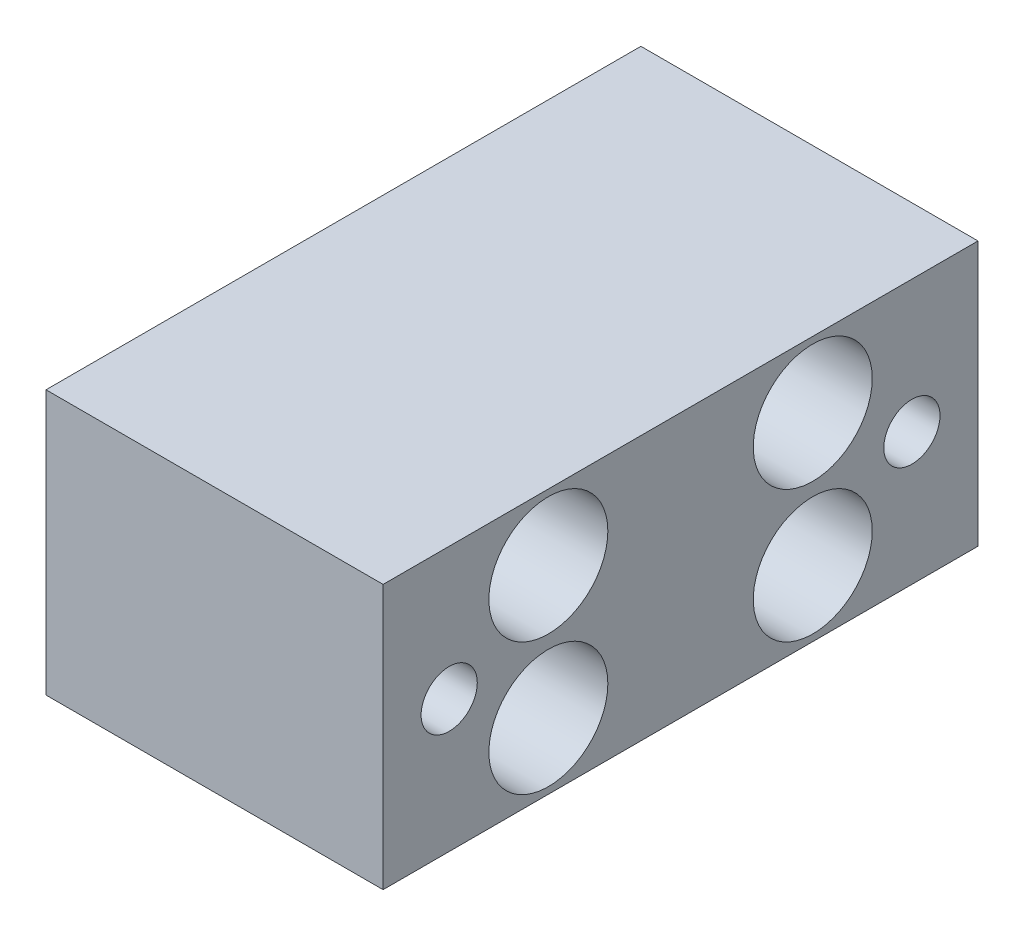
SolidWorks part; units mm, degrees
ref_plane "前视基准面" through (0, 0, 0) normal (0, 0, 1) x (1, 0, 0)
ref_plane "上视基准面" through (0, 0, 0) normal (0, 1, 0) x (1, 0, 0)
ref_plane "右视基准面" through (0, 0, 0) normal (1, 0, 0) x (0, 0, -1)
sketch "草图1" plane through (0, 0, 0) normal (1, 0, 0) x (0, 0, -1)
  line L1 (-45, 20) -> (45, 20)
  line L2 (-45, 20) -> (-45, -20)
  line L3 (-45, -20) -> (45, -20)
  line L4 (45, 20) -> (45, -20)
  line L5 (-45, 20) -> (45, -20) construction
  line L6 (-45, -20) -> (45, 20) construction
  point P0 (0, 0)
  dimension "D1" = 90
  dimension "D2" = 40
extrude "凸台-拉伸1" add sketch "草图1" along normal blind 51
hole_wizard "打孔尺寸(%根据)内六角圆柱头螺钉的类型1" positions "草图2" profile "草图3" counterbore size "M10" standard "GB" end condition through all
sketch "草图2" plane through (51, 0, 0) normal (1, 0, 0) x (0, 0, -1)
  line L0 (0, 34.8993) -> (0, 0) construction
  line L1 (0, 0) -> (67.0588, 0) construction
  point P0 (-20, 10)
  point P2 (20, 10)
  point P4 (-20, -10)
  point P6 (20, -10)
  dimension "D1" = 40
  dimension "D2" = 20
sketch "草图3" plane through (51, 10, 20) normal (0, 1, 0) x (0, 0, -1)
  line L0 (0, 0) -> (0, 51)
  line L1 (0, 51) -> (5.5, 51)
  line L3 (5.5, 51) -> (5.5, 40)
  line L4 (5.5, 40) -> (9, 40)
  line L5 (9, 40) -> (9, 0)
  line L7 (9, 0) -> (0, 0)
  line L11 (0, -6.35) -> (0, 107.95) construction
  dimension "通孔孔直径" = 11
  dimension "通孔孔深度" = 51
  dimension "柱形沉头孔直径" = 18
  dimension "柱形沉头孔深度" = 40
hole_wizard "M10 螺纹孔1" positions "草图4" profile "草图5" tap size "M10" standard "GB"
sketch "草图4" plane through (51, 0, 0) normal (1, 0, 0) x (0, 0, -1)
  line L0 (0, 0) -> (53.5427, 0) construction
  line L2 (0, 0) -> (0, 29.0414) construction
  point P0 (-35, 0)
  point P2 (35, 0)
  dimension "D1" = 70
sketch "草图5" plane through (51, 0, 35) normal (0, 1, 0) x (0, 0, -1)
  line L0 (0, 0) -> (0, 27.0537)
  line L1 (0, 27.0537) -> (4.25, 24.5)
  line L2 (4.25, 24.5) -> (4.25, 0)
  line L5 (4.25, 0) -> (0, 0)
  line L10 (0, 27.0537) -> (-4.25, 24.5) construction
  line L11 (0, -6.35) -> (0, 107.95) construction
  dimension "螺纹孔钻头直径" = 8.5
  dimension "螺纹孔钻头深度" = 24.5
  dimension "导头角度" = 118
cosmetic thread "孔螺蚊线1"
cosmetic thread "孔螺蚊线2"
